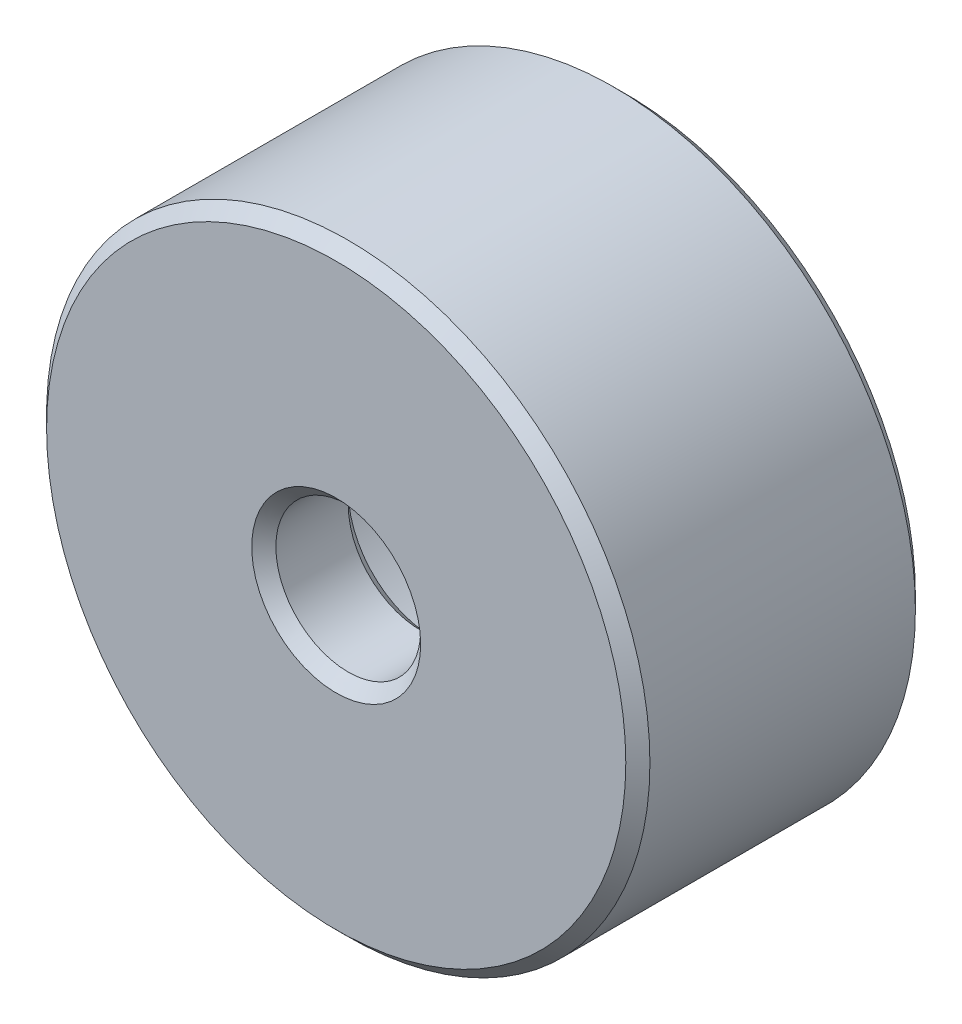
SolidWorks part; units mm, degrees
ref_plane "Front Plane" through (0, 0, 0) normal (0, 0, 1) x (1, 0, 0)
ref_plane "Top Plane" through (0, 0, 0) normal (0, 1, 0) x (1, 0, 0)
ref_plane "Right Plane" through (0, 0, 0) normal (1, 0, 0) x (0, 0, -1)
sketch "Sketch1" plane through (0, 0, 0) normal (0, 0, 1) x (1, 0, 0)
  circle A0 centre (0, 0) radius 3
  circle A1 centre (0, 0) radius 12.5
  dimension "D1" = 6
  dimension "D2" = 25
extrude "Boss-Extrude1" add sketch "Sketch1" along normal mid plane 12
sketch "Sketch2" plane through (0, 0, -6) normal (0, 0, -1) x (-1, 0, 0)
  circle A0 centre (0, 0) radius 8
  dimension "D1" = 16
extrude "Cut-Extrude1" cut sketch "Sketch2" against normal blind 8
chamfer "Chamfer1" distance 0.5 angle 45 5 edges at (3, 0, 6) (-3, 0, 2) (-8, 0, -6) (12.5, 0, 6) (12.5, 0, -6)
